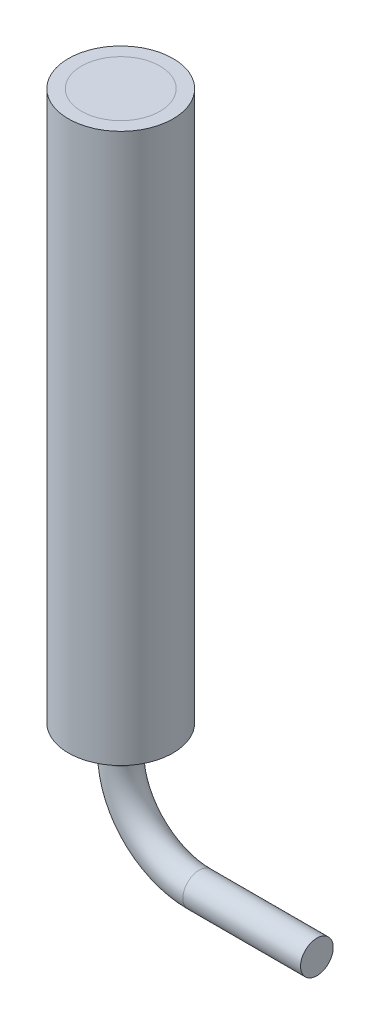
from build123d import *

# Parameters (mm, degrees)
SKETCH1_R           = 4
BOSS_EXTRUDE1_DEPTH = 42
SKETCH2_R           = 1.25


with BuildPart() as part:
    # Sketch1 → Boss-Extrude1 (new body)
    with BuildSketch(Plane(origin=(0, 0, 0), x_dir=(1, 0, 0), z_dir=(0, 1, 0))):
        with Locations(Location((0, 0, 0), (0, 0, 90))):
            Circle(SKETCH1_R)
    extrude(amount=BOSS_EXTRUDE1_DEPTH)

    # Sweep1: sweep along a path in Sketch3
    with BuildLine(Plane.XY) as sweep1_path:
        Line((0, 0), (0, -2))
        ThreePointArc((0, -2), (1.757359313, -6.242640687), (6, -8))
        Line((6, -8), (15, -8))
    # Sketch2 → Sweep1 (sweep)
    with BuildSketch(Plane.XZ):
        Circle(SKETCH2_R)
    sweep(path=sweep1_path.line)


solid = part.part
